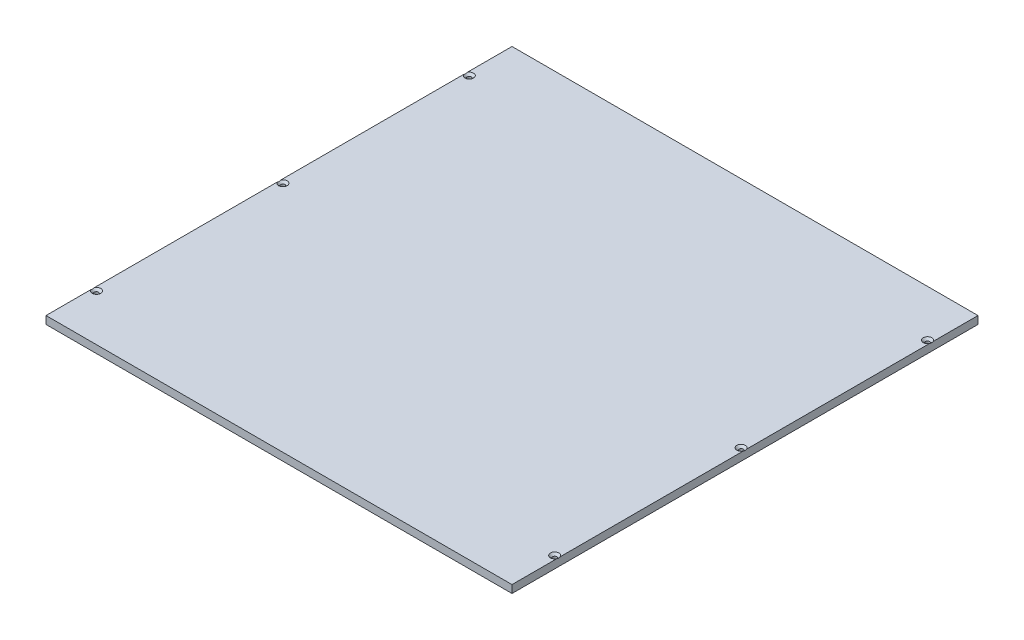
SolidWorks part; units mm, degrees
ref_plane "Front Plane" through (0, 0, 0) normal (0, 0, 1) x (1, 0, 0)
ref_plane "Top Plane" through (0, 0, 0) normal (0, 1, 0) x (1, 0, 0)
ref_plane "Right Plane" through (0, 0, 0) normal (1, 0, 0) x (0, 0, -1)
sketch "Sketch1" plane through (0, 0, 0) normal (0, 1, 0) x (1, 0, 0)
  line L1 (-150, -150) -> (150, -150)
  line L2 (-150, -150) -> (-150, 150)
  line L3 (-150, 150) -> (150, 150)
  line L4 (150, -150) -> (150, 150)
  line L5 (-150, -150) -> (150, 150) construction
  line L6 (-150, 150) -> (150, -150) construction
  point P0 (0, 0)
  dimension "D1" = 300
  dimension "D2" = 300
extrude "Boss-Extrude1" add sketch "Sketch1" along normal blind 5
hole_wizard "CSK for M2.5 Flat Head Machine Screw1" positions "Sketch2" profile "Sketch3" countersink size "M2.5" standard "ANSI Metric"
sketch "Sketch2" plane through (0, 5, 0) normal (0, 1, 0) x (1, 0, 0)
  line L0 (150, -150) -> (150, 150) construction
  line L1 (-150, 150) -> (-150, -150) construction
  point P0 (147.5, 120)
  point P2 (147.5, 0)
  point P4 (147.5, -120)
  point P6 (-147.5, 120)
  point P8 (-147.5, 0)
  point P10 (-147.5, -120)
  dimension "D1" = 2.5
  dimension "D2" = 2.5
  dimension "D3" = 2.5
  dimension "D4" = 2.5
  dimension "D5" = 2.5
  dimension "D6" = 2.5
  dimension "D7" = 0
  dimension "D8" = 120
  dimension "D9" = 120
  dimension "D10" = 0
  dimension "D11" = 120
  dimension "D12" = 120
sketch "Sketch3" plane through (147.5, 5, -120) normal (1, 0, 0) x (0, 0, 1)
  line L0 (0, 0) -> (0, 17.8112)
  line L1 (0, 17.8112) -> (1.35, 17)
  line L2 (1.35, 17) -> (1.35, 1.4)
  line L3 (1.35, 1.4) -> (2.75, 0)
  line L5 (2.75, 0) -> (0, 0)
  line L6 (-1.35, 1.4) -> (-2.75, 0) construction
  line L10 (0, 17.8112) -> (-1.35, 17) construction
  line L11 (0, -6.35) -> (0, 107.95) construction
  dimension "孔直径" = 2.7
  dimension "孔深度" = 17
  dimension "近端锥形沉头孔直径" = 5.5
  dimension "近端锥形沉头孔角度" = 90
  dimension "导头角度" = 118
